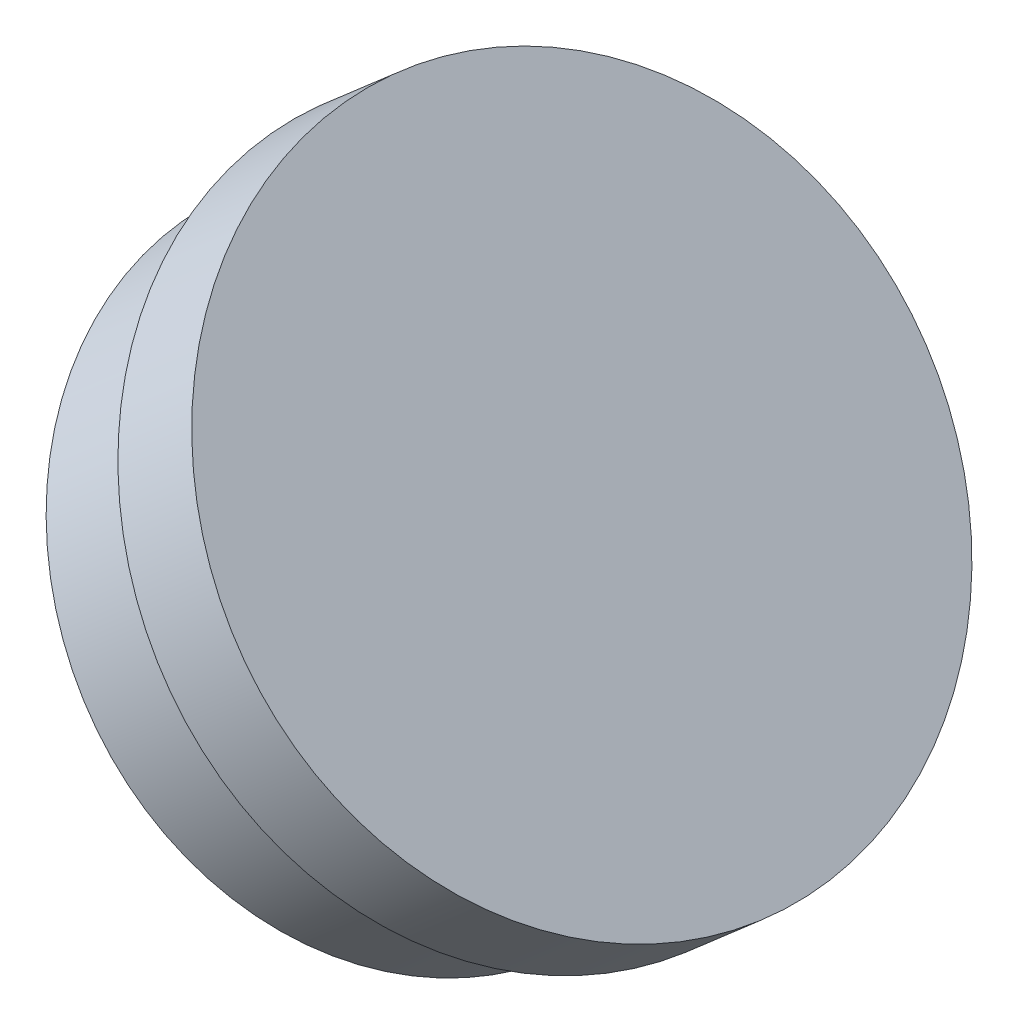
SolidWorks part; units mm, degrees
material "20#"
ref_plane "Front Plane" through (0, 0, 0) normal (0, 0, 1) x (1, 0, 0)
ref_plane "Top Plane" through (0, 0, 0) normal (0, 1, 0) x (1, 0, 0)
ref_plane "Right Plane" through (0, 0, 0) normal (1, 0, 0) x (0, 0, -1)
sketch "Sketch1" plane through (0, 0, 0) normal (0, 0, 1) x (1, 0, 0)
  line L0 (1431.4933, -44.9822) -> (1430.8372, -44.2275)
  line L1 (1434.1175, -48.001) -> (1427.5569, -40.4539) construction
  line L2 (1430.8372, -44.2275) -> (1433.1013, -42.2593)
  line L3 (1433.1013, -42.2593) -> (1439.6619, -49.8064)
  line L4 (1439.6619, -49.8064) -> (1434.9827, -53.874) construction
  line L5 (1431.0464, -49.3457) -> (1546.7523, -182.4501) construction
  line L6 (1431.4933, -44.9822) -> (1430.2857, -46.0319) construction
  line L7 (1431.4933, -44.9822) -> (1427.7197, -48.2625)
  line L8 (1427.7197, -48.2625) -> (1433.6242, -55.0549)
  line L9 (1433.6242, -55.0549) -> (1439.6619, -49.8064)
  dimension "D1" = 9
  dimension "D2" = 5
  dimension "D3" = 3
  dimension "D4" = 10
  dimension "D5" = 9
revolve "Revolve1" add sketch "Sketch1" angle 360 about L4
chamfer "Chamfer1" distance 0.5 angle 45 1 edges at (1427.7197, -48.2625, 0)
